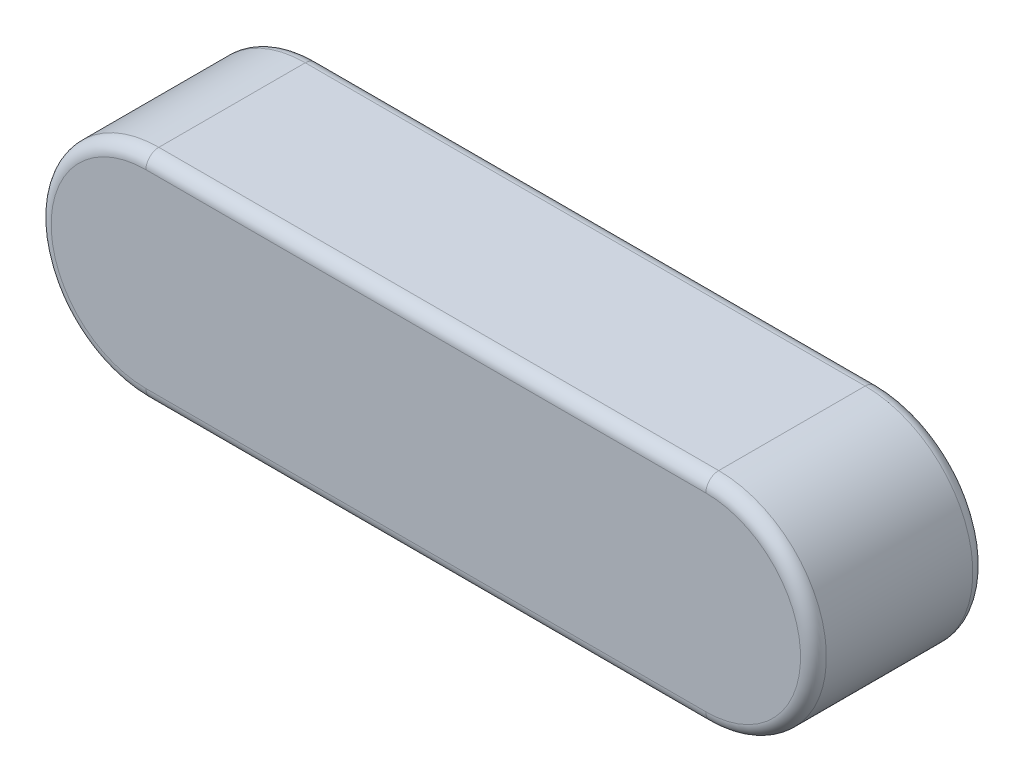
SolidWorks part; units mm, degrees
material "45"
ref_plane "基准面1" through (0, 0, 0) normal (0, 0, 1) x (1, 0, 0)
ref_plane "基准面2" through (0, 0, 0) normal (0, 1, 0) x (1, 0, 0)
ref_plane "基准面3" through (0, 0, 0) normal (1, 0, 0) x (0, 0, -1)
sketch "尺寸草图" plane through (0, 0, 0) normal (0, 0, 1) x (1, 0, 0)
  line L0 (-16, 0) -> (16, 0) construction
  point P3 (-8, 0)
  point P4 (-0.6, 0)
  point P5 (0, 0)
  point P8 (-10, 0)
  point P11 (0, 0)
sketch "草图1" plane through (0, 0, 0) normal (0, 0, 1) x (1, 0, 0)
  line L0 (-28.0599, 0) -> (30.562, 0) construction
  line L1 (-13, 5) -> (13, 5)
  line L2 (-13, -5) -> (13, -5)
  line L3 (0, 2.9108) -> (0, -2.1805) construction
  arc A0 (-13, 5) -> (-13, -5) centre (-13, 0) ccw
  arc A1 (13, 5) -> (13, -5) centre (13, 0) cw
extrude "基体-拉伸" add sketch "草图1" along normal blind 8
fillet "圆角1" radius 0.6 8 edges at (18, 0, 8) (0, 5, 8) (-18, 0, 8) (0, 5, 0) (18, 0, 0) (0, -5, 0) (-18, 0, 0) (0, -5, 8)
equation "\"D1@草图1\" = \"b@尺寸草图\" / 2"
equation "\"D1@圆角1\" = \"r@尺寸草图\""
equation "\"D1@基体-拉伸\" = \"h@尺寸草图\""
